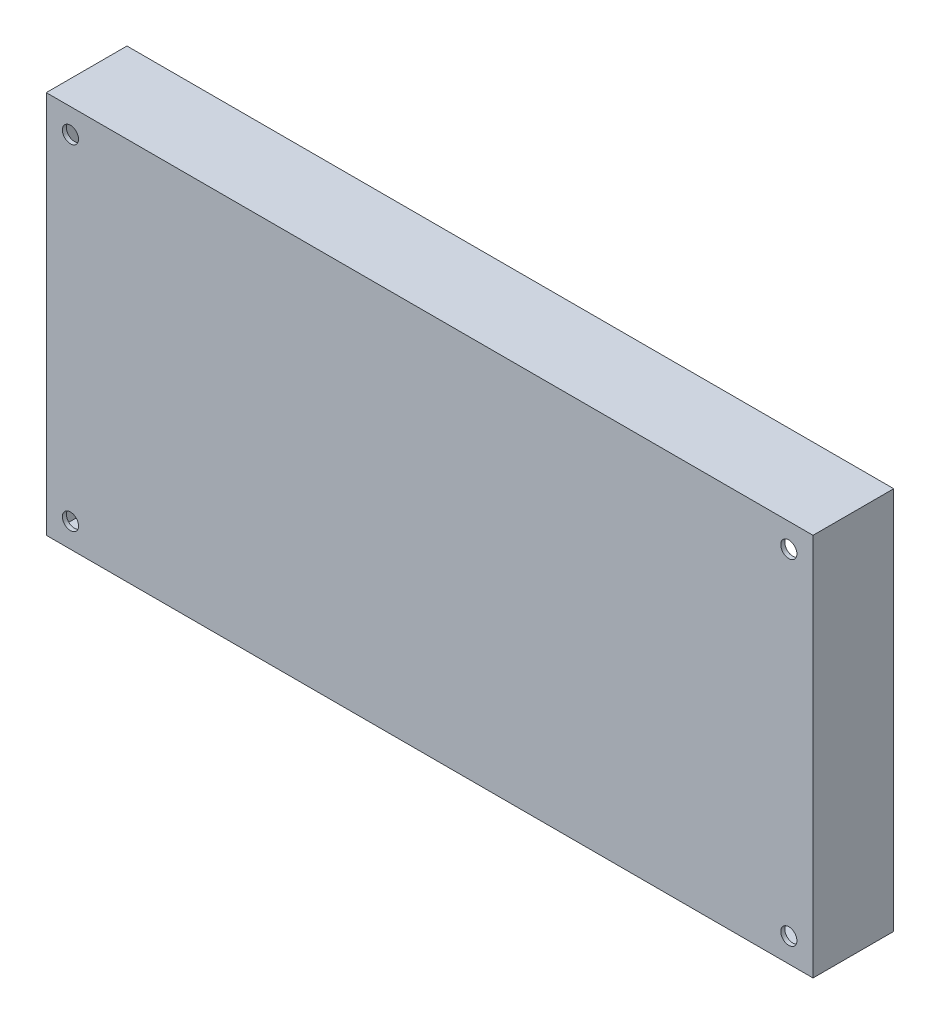
SolidWorks part; units mm, degrees
ref_plane "Front Plane" through (0, 0, 0) normal (0, 0, 1) x (1, 0, 0)
ref_plane "Top Plane" through (0, 0, 0) normal (0, 1, 0) x (1, 0, 0)
ref_plane "Right Plane" through (0, 0, 0) normal (1, 0, 0) x (0, 0, -1)
other "Configuration Table"
sketch "Sketch1" plane through (0, 0, 0) normal (0, 0, 1) x (1, 0, 0)
  line L1 (-27.8614, 85.6253) -> (162.1386, 85.6253)
  line L2 (-27.8614, 85.6253) -> (-27.8614, -9.3747)
  line L3 (-27.8614, -9.3747) -> (162.1386, -9.3747)
  line L4 (162.1386, 85.6253) -> (162.1386, -9.3747)
extrude "Boss-Extrude1" add sketch "Sketch1" along normal blind 20
shell "Shell1" thickness 1
sketch "Sketch2" plane through (0, 85.6253, 0) normal (0, 1, 0) x (1, 0, 0)
  line L0 (139.1386, -9) -> (139.1386, -8)
  line L2 (139.1386, -8) -> (139.6386, -8)
  line L3 (139.1386, -19) -> (139.6386, -19)
  line L4 (-19.8614, -19) -> (126.1386, -19)
  line L5 (-19.8614, -19) -> (-19.8614, -9)
  line L6 (-19.8614, -9) -> (126.1386, -9)
  line L7 (126.1386, -19) -> (126.1386, -9)
  line L9 (127.1386, -19) -> (139.1386, -19)
  line L10 (127.1386, -19) -> (127.1386, -9)
  line L11 (127.1386, -9) -> (139.1386, -9)
  line L14 (139.6386, -19) -> (149.6386, -19)
  line L16 (139.6386, -8) -> (149.6386, -8)
  line L17 (149.6386, -19) -> (149.6386, -8)
extrude "Cut-Extrude1" cut sketch "Sketch2" against normal blind 1
sketch "Sketch4" plane through (0, -9.3747, 0) normal (0, -1, 0) x (1, 0, 0)
  line L0 (124.1661, 9.8517) -> (138.1661, 9.8517)
  line L3 (-17.8339, 9.8517) -> (-14.8339, 9.8517)
  line L4 (-17.8339, 19) -> (138.1661, 19)
  line L5 (-17.8339, 19) -> (-17.8339, 9.8517)
  line L7 (138.1661, 19) -> (138.1661, 9.8517)
  line L8 (-11.8339, 9.8517) -> (5.1661, 9.8517)
  line L10 (-14.8339, 9.8517) -> (-14.8339, 7.8517)
  line L11 (-14.8339, 7.8517) -> (-11.8339, 7.8517)
  line L12 (-11.8339, 9.8517) -> (-11.8339, 7.8517)
  line L13 (8.1661, 9.8517) -> (14.1661, 9.8517)
  line L15 (5.1661, 9.8517) -> (5.1661, 7.8517)
  line L16 (5.1661, 7.8517) -> (8.1661, 7.8517)
  line L17 (8.1661, 9.8517) -> (8.1661, 7.8517)
  line L18 (17.1661, 9.8517) -> (34.1661, 9.8517)
  line L20 (14.1661, 9.8517) -> (14.1661, 7.8517)
  line L21 (14.1661, 7.8517) -> (17.1661, 7.8517)
  line L22 (17.1661, 9.8517) -> (17.1661, 7.8517)
  line L23 (37.1661, 9.8517) -> (43.1661, 9.8517)
  line L25 (34.1661, 9.8517) -> (34.1661, 7.8517)
  line L26 (34.1661, 7.8517) -> (37.1661, 7.8517)
  line L27 (37.1661, 9.8517) -> (37.1661, 7.8517)
  line L28 (46.1661, 9.8517) -> (63.1661, 9.8517)
  line L30 (43.1661, 9.8517) -> (43.1661, 7.8517)
  line L31 (43.1661, 7.8517) -> (46.1661, 7.8517)
  line L32 (46.1661, 9.8517) -> (46.1661, 7.8517)
  line L33 (66.1661, 9.8517) -> (72.1661, 9.8517)
  line L35 (63.1661, 9.8517) -> (63.1661, 7.8517)
  line L36 (63.1661, 7.8517) -> (66.1661, 7.8517)
  line L37 (66.1661, 9.8517) -> (66.1661, 7.8517)
  line L38 (75.1661, 9.8517) -> (92.1661, 9.8517)
  line L40 (72.1661, 9.8517) -> (72.1661, 7.8517)
  line L41 (72.1661, 7.8517) -> (75.1661, 7.8517)
  line L42 (75.1661, 9.8517) -> (75.1661, 7.8517)
  line L43 (95.1661, 9.8517) -> (101.1661, 9.8517)
  line L45 (92.1661, 9.8517) -> (92.1661, 7.8517)
  line L46 (92.1661, 7.8517) -> (95.1661, 7.8517)
  line L47 (95.1661, 9.8517) -> (95.1661, 7.8517)
  line L48 (104.1661, 9.8517) -> (121.1661, 9.8517)
  line L50 (101.1661, 9.8517) -> (101.1661, 7.8517)
  line L51 (101.1661, 7.8517) -> (104.1661, 7.8517)
  line L52 (104.1661, 9.8517) -> (104.1661, 7.8517)
  line L55 (121.1661, 9.8517) -> (121.1661, 7.8517)
  line L56 (121.1661, 7.8517) -> (124.1661, 7.8517)
  line L57 (124.1661, 9.8517) -> (124.1661, 7.8517)
  line L60 (105.1661, 6.8517) -> (114.1661, 6.8517)
  line L61 (105.1661, 6.8517) -> (105.1661, 1.7841)
  line L62 (105.1661, 1.7841) -> (114.1661, 1.7841)
  line L63 (114.1661, 6.8517) -> (114.1661, 1.7841)
  circle A0 centre (144.1386, 6.5) radius 3.5
extrude "Cut-Extrude2" cut sketch "Sketch4" against normal blind 10
sketch "Sketch5" plane through (0, 85.6253, 0) normal (0, 1, 0) x (1, 0, 0)
  line L0 (-13.8614, -9) -> (-16.8614, -9)
  line L1 (126.1386, -9) -> (-19.8614, -9) construction
  line L4 (-16.8614, -9) -> (-16.8614, -7)
  line L5 (-16.8614, -7) -> (-13.8614, -7)
  line L6 (-13.8614, -9) -> (-13.8614, -7)
  line L8 (13.1386, -9) -> (16.1386, -9)
  line L9 (13.1386, -9) -> (13.1386, -7)
  line L10 (13.1386, -7) -> (16.1386, -7)
  line L11 (16.1386, -9) -> (16.1386, -7)
  line L13 (23.1386, -9) -> (26.1386, -9)
  line L14 (23.1386, -9) -> (23.1386, -7)
  line L15 (23.1386, -7) -> (26.1386, -7)
  line L16 (26.1386, -9) -> (26.1386, -7)
  line L18 (53.1386, -9) -> (56.1386, -9)
  line L19 (53.1386, -9) -> (53.1386, -7)
  line L20 (53.1386, -7) -> (56.1386, -7)
  line L21 (56.1386, -9) -> (56.1386, -7)
  line L23 (63.1386, -9) -> (66.1386, -9)
  line L24 (63.1386, -9) -> (63.1386, -7)
  line L25 (63.1386, -7) -> (66.1386, -7)
  line L26 (66.1386, -9) -> (66.1386, -7)
  line L28 (83.1386, -9) -> (86.1386, -9)
  line L29 (83.1386, -9) -> (83.1386, -7)
  line L30 (83.1386, -7) -> (86.1386, -7)
  line L31 (86.1386, -9) -> (86.1386, -7)
  line L33 (93.1386, -9) -> (96.1386, -9)
  line L34 (93.1386, -9) -> (93.1386, -7)
  line L35 (93.1386, -7) -> (96.1386, -7)
  line L36 (96.1386, -9) -> (96.1386, -7)
  line L38 (113.1386, -9) -> (116.1386, -9)
  line L39 (113.1386, -9) -> (113.1386, -7)
  line L40 (113.1386, -7) -> (116.1386, -7)
  line L41 (116.1386, -9) -> (116.1386, -7)
extrude "Cut-Extrude3" cut sketch "Sketch5" against normal blind 1
sketch "Sketch6" plane through (0, 0, 20) normal (0, 0, 1) x (1, 0, 0)
  circle A0 centre (-21.8614, -3.3747) radius 2
  circle A1 centre (-21.8614, 79.6253) radius 2
  circle A2 centre (156.1386, 79.6253) radius 2
  circle A3 centre (156.1386, -3.3747) radius 2
extrude "Cut-Extrude4" cut sketch "Sketch6" against normal blind 1
sketch "Sketch8" plane through (0, 85.6253, 0) normal (0, 1, 0) x (1, 0, 0)
  line L0 (16.1386, -9) -> (16.1386, -7) construction
  line L1 (-19.8614, -9) -> (-16.8614, -9)
  line L2 (-19.8614, -9) -> (-19.8614, -7)
  line L3 (-19.8614, -7) -> (-16.8614, -7)
  line L4 (-16.8614, -9) -> (-16.8614, -7)
  line L5 (-13.8614, -9) -> (13.1386, -9)
  line L6 (-13.8614, -9) -> (-13.8614, -7)
  line L7 (-13.8614, -7) -> (13.1386, -7)
  line L8 (13.1386, -9) -> (13.1386, -7)
  line L9 (16.1386, -9) -> (23.1386, -9)
  line L10 (16.1386, -9) -> (16.1386, -7)
  line L11 (16.1386, -7) -> (23.1386, -7)
  line L12 (23.1386, -9) -> (23.1386, -7)
  line L13 (23.1386, -9) -> (16.1386, -9) construction
  line L14 (53.1386, -9) -> (26.1386, -9) construction
  line L15 (26.1386, -9) -> (53.1386, -9)
  line L16 (26.1386, -9) -> (26.1386, -7)
  line L17 (26.1386, -7) -> (53.1386, -7)
  line L18 (53.1386, -9) -> (53.1386, -7)
  line L19 (53.1386, -7) -> (53.1386, -9) construction
  line L21 (56.1386, -9) -> (63.1386, -9)
  line L22 (56.1386, -9) -> (56.1386, -7)
  line L23 (56.1386, -7) -> (63.1386, -7)
  line L24 (63.1386, -9) -> (63.1386, -7)
  line L25 (66.1386, -9) -> (83.1386, -9)
  line L26 (66.1386, -9) -> (66.1386, -7)
  line L27 (66.1386, -7) -> (83.1386, -7)
  line L28 (83.1386, -9) -> (83.1386, -7)
  line L29 (86.1386, -9) -> (93.1386, -9)
  line L30 (86.1386, -9) -> (86.1386, -7)
  line L31 (86.1386, -7) -> (93.1386, -7)
  line L32 (93.1386, -9) -> (93.1386, -7)
  line L33 (96.1386, -9) -> (113.1386, -9)
  line L34 (96.1386, -9) -> (96.1386, -7)
  line L35 (96.1386, -7) -> (113.1386, -7)
  line L36 (113.1386, -9) -> (113.1386, -7)
  line L37 (116.1386, -9) -> (126.1386, -9)
  line L38 (116.1386, -9) -> (116.1386, -7)
  line L39 (116.1386, -7) -> (126.1386, -7)
  line L40 (126.1386, -9) -> (126.1386, -7)
extrude "Cut-Extrude5" cut sketch "Sketch8" against normal blind 1
sketch "Sketch9" plane through (0, -9.3747, 0) normal (0, -1, 0) x (1, 0, 0)
  line L1 (-17.8339, 9.8517) -> (-14.8339, 9.8517)
  line L2 (-17.8339, 9.8517) -> (-17.8339, 7.8517)
  line L3 (-17.8339, 7.8517) -> (-14.8339, 7.8517)
  line L4 (-14.8339, 9.8517) -> (-14.8339, 7.8517)
  line L5 (-11.8339, 9.8517) -> (5.1661, 9.8517)
  line L6 (-11.8339, 9.8517) -> (-11.8339, 7.8517)
  line L7 (-11.8339, 7.8517) -> (5.1661, 7.8517)
  line L8 (5.1661, 9.8517) -> (5.1661, 7.8517)
  line L9 (8.1661, 9.8517) -> (14.1661, 9.8517)
  line L10 (8.1661, 9.8517) -> (8.1661, 7.8517)
  line L11 (8.1661, 7.8517) -> (14.1661, 7.8517)
  line L12 (14.1661, 9.8517) -> (14.1661, 7.8517)
  line L13 (17.1661, 9.8517) -> (34.1661, 9.8517)
  line L14 (17.1661, 9.8517) -> (17.1661, 7.8517)
  line L15 (17.1661, 7.8517) -> (34.1661, 7.8517)
  line L16 (34.1661, 9.8517) -> (34.1661, 7.8517)
  line L17 (37.1661, 9.8517) -> (43.1661, 9.8517)
  line L18 (37.1661, 9.8517) -> (37.1661, 7.8517)
  line L19 (37.1661, 7.8517) -> (43.1661, 7.8517)
  line L20 (43.1661, 9.8517) -> (43.1661, 7.8517)
  line L21 (46.1661, 9.8517) -> (63.1661, 9.8517)
  line L22 (46.1661, 9.8517) -> (46.1661, 7.8517)
  line L23 (46.1661, 7.8517) -> (63.1661, 7.8517)
  line L24 (63.1661, 9.8517) -> (63.1661, 7.8517)
  line L25 (66.1661, 9.8517) -> (72.1661, 9.8517)
  line L26 (66.1661, 9.8517) -> (66.1661, 7.8517)
  line L27 (66.1661, 7.8517) -> (72.1661, 7.8517)
  line L28 (72.1661, 9.8517) -> (72.1661, 7.8517)
  line L29 (75.1661, 9.8517) -> (92.1661, 9.8517)
  line L30 (75.1661, 9.8517) -> (75.1661, 7.8517)
  line L31 (75.1661, 7.8517) -> (92.1661, 7.8517)
  line L32 (92.1661, 9.8517) -> (92.1661, 7.8517)
  line L33 (95.1661, 9.8517) -> (101.1661, 9.8517)
  line L34 (95.1661, 9.8517) -> (95.1661, 7.8517)
  line L35 (95.1661, 7.8517) -> (101.1661, 7.8517)
  line L36 (101.1661, 9.8517) -> (101.1661, 7.8517)
  line L37 (104.1661, 9.8517) -> (121.1661, 9.8517)
  line L38 (104.1661, 9.8517) -> (104.1661, 7.8517)
  line L39 (104.1661, 7.8517) -> (121.1661, 7.8517)
  line L40 (121.1661, 9.8517) -> (121.1661, 7.8517)
  line L41 (124.1661, 9.8517) -> (138.1661, 9.8517)
  line L42 (124.1661, 9.8517) -> (124.1661, 7.8517)
  line L43 (124.1661, 7.8517) -> (138.1661, 7.8517)
  line L44 (138.1661, 9.8517) -> (138.1661, 7.8517)
extrude "Cut-Extrude6" cut sketch "Sketch9" against normal blind 1
sketch "Sketch10" plane through (0, 85.6253, 0) normal (0, 1, 0) x (1, 0, 0)
  line L1 (-19.8614, -7) -> (126.1386, -7)
  line L2 (-19.8614, -7) -> (-19.8614, -19)
  line L3 (-19.8614, -19) -> (126.1386, -19)
  line L4 (126.1386, -7) -> (126.1386, -19)
extrude "Boss-Extrude2" add sketch "Sketch10" against normal blind 1
sketch "Sketch11" plane through (0, -9.3747, 0) normal (0, -1, 0) x (1, 0, 0)
  line L1 (-17.8339, 19) -> (138.1661, 19)
  line L2 (-17.8339, 19) -> (-17.8339, 7.8517)
  line L3 (-17.8339, 7.8517) -> (138.1661, 7.8517)
  line L4 (138.1661, 19) -> (138.1661, 7.8517)
  line L5 (105.1661, 6.8517) -> (114.1661, 6.8517)
  line L6 (105.1661, 6.8517) -> (105.1661, 1.7841)
  line L7 (105.1661, 1.7841) -> (114.1661, 1.7841)
  line L8 (114.1661, 6.8517) -> (114.1661, 1.7841)
  circle A0 centre (144.1386, 6.5) radius 3.5
extrude "Boss-Extrude3" add sketch "Sketch11" against normal blind 1
sketch "Sketch12" plane through (0, 85.6253, 0) normal (0, 1, 0) x (1, 0, 0)
  line L1 (149.6386, -8) -> (127.1386, -8)
  line L2 (149.6386, -8) -> (149.6386, -19)
  line L3 (149.6386, -19) -> (127.1386, -19)
  line L4 (127.1386, -8) -> (127.1386, -19)
extrude "Boss-Extrude4" add sketch "Sketch12" against normal blind 1
